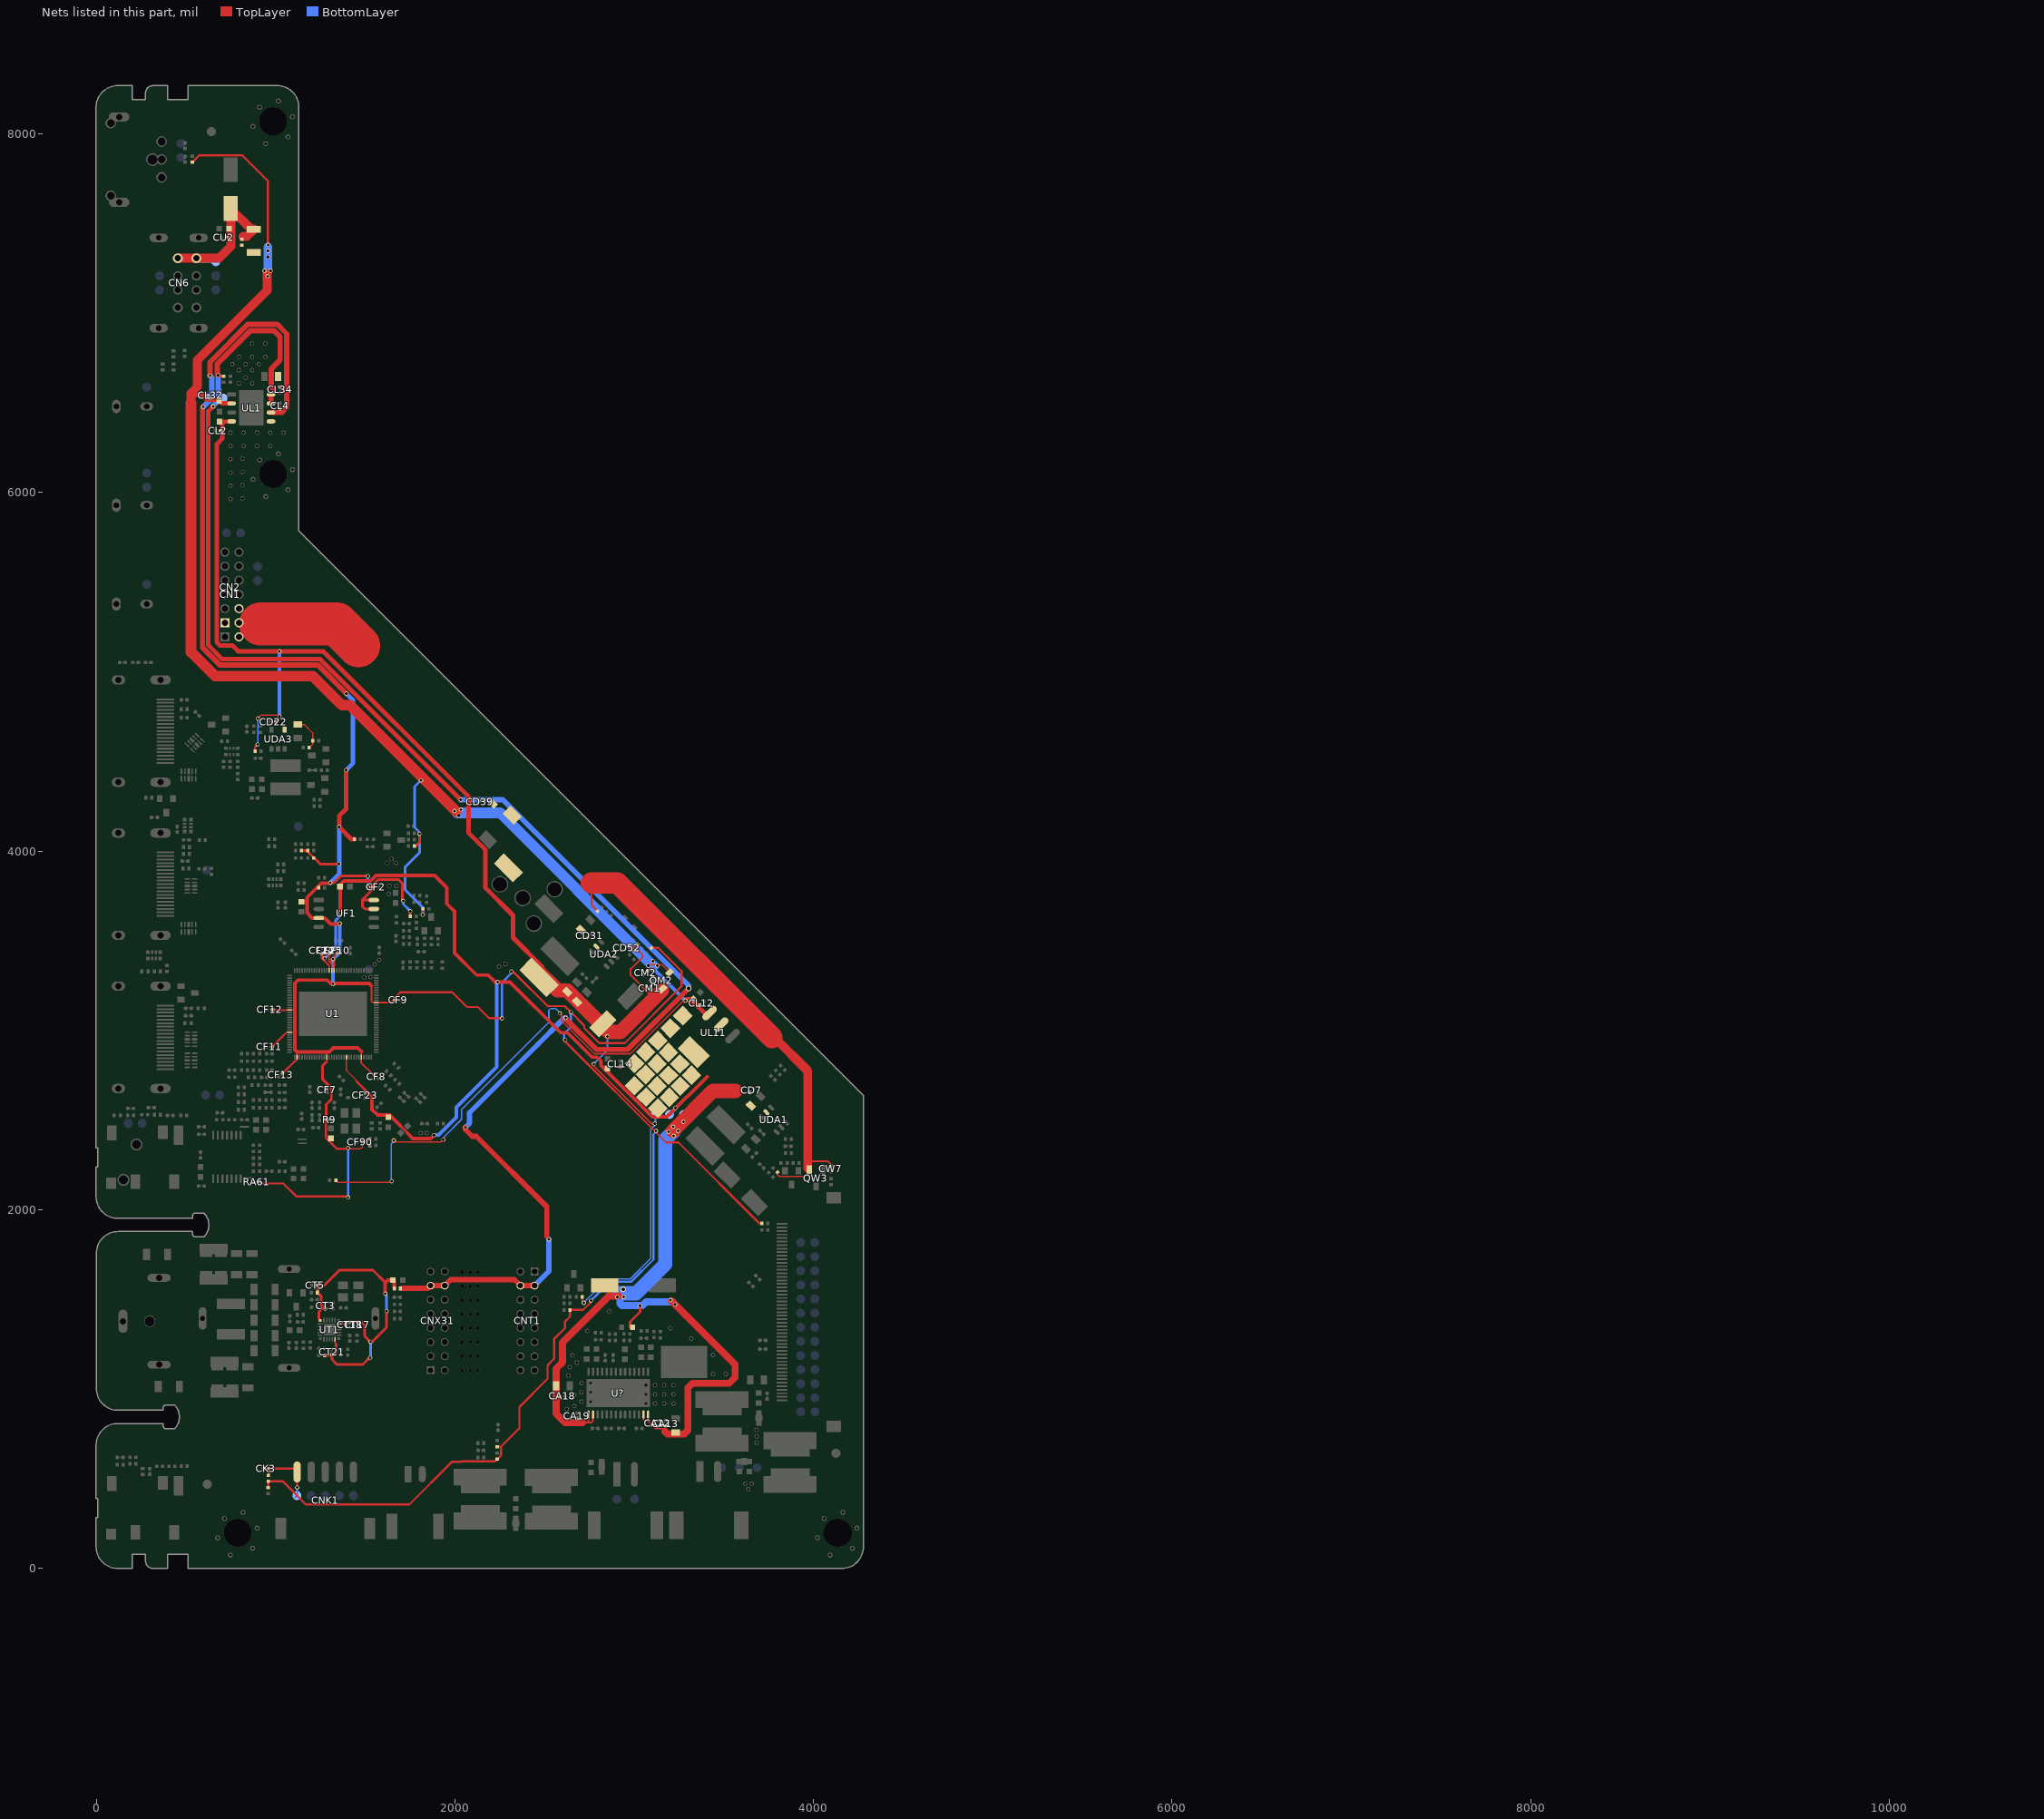
[diagram p0: the nets of this part, all layers, seen from the top]
# Altium PCB MISC105950.PcbDoc (part 5 of 15)
Units mil, origin at the board's own origin, x right, y up, seen from the top; angles counter-clockwise.
Board outline 4280.62 x 8272.76 mil, 2 copper layers (TopLayer, BottomLayer), stack 61.855 mil thick; 541 components, 268 nets, 2324 pads, 1157 vias.

## Part data (continued)
RD43: library part 1K5ohm-0402-±1%-1/16W-D
RD81: library part 10Kohm-0402-±1%-1/16W-D
RD88: library part 12Kohm-0402-±1%-1/16W-D
RF3 RF13 RF29 RF43 RF44 RG3 RG29 RK25 RW13: library part 4K7ohm-0402-±5%-1/16W-D
RF4: library part 100ohm-0402-±5%-1/16W-
RF5: library part 1Kohm-0402-±5%-1/16W-
RF12 RF19 RH101 RH102 RH103 RH104 RH105 RH106: library part 68ohm-0402-±5%-1/16W-D
RFT1: library part XXX.XXX.0005128-D, "RF connector, RF JACK, H, IEC, T14.5, CH6.3, with pipe, 23.8×15.1×11.9mm, SMD, 120-XX1, GD-D"
RG6 RG7 RH72 RH73: library part 33ohm-0402-±5%-1/16W-D
RG8 RG9 RG66 RG67 RH23 RH33 RH70 RK6 RK23: library part 1Kohm-0402-±5%-1/16W-D
RH1 RH74 RH81: library part 22Kohm-0402-±5%-1/16W-D
RH2 RH75 RH82: library part 33Kohm-0402-±5%-1/16W-D
RH24 RH34 RH35 RH71: library part 4*100ohm-0402-±5%-1/16W-D
RH83 RO22 RT1 RT2 RT3 RT4 RT5: library part 004.002.0000568-D, "Thick-film resistor, RES, 1/16W, 100ohm, ±5%, 0402, SMD-D"
RI14 RI16: library part 12Kohm-0402-±5%-1/16W-D
RI21 RI23 RI25 RI36: library part 004.002.0000728-D, "Thick-film resistor, RES, 1/16W, 75ohm, ±5%, 0402, SMD-D"
RI22 RI24 RI26 RI38: library part 004.002.0000658-D, "Thick-film resistor, RES, 1/16W, 33ohm, ±5%, 0402, SMD-D"
RI62 RI63: library part 150ohm-0402-±5%-1/16W-D
RK1: library part 33ohm-0402-±5%-1/16W-
RK2: library part 4K7ohm-0402-±1%-1/16W-D
RK13: library part 004.002.0000663-D, "Thick-film resistor, RES, 1/16W, 33Kohm, ±5%, 0402, SMD-D"
RK14: library part 004.002.0000699-D, "Thick-film resistor, RES, 1/16W, 510ohm, ±1%, 0402, SMD-D"
RL31: library part 004.002.0000584-D, "Thick-film resistor, RES, 1/16W, 120ohm, ±1%, 0402, SMD-D"
RL32: library part 004.002.0000616-D, "Thick-film resistor, RES, 1/16W, 200ohm, ±1%, 0402, SMD-D"
RO21: library part 004.002.0000609-D, "Thick-film resistor, RES, 1/16W, 180ohm, ±5%, 0402, SMD-D"
RO31 RU1: library part 004.002.0000558-D, "Thick-film resistor, RES, 1/16W, 0ohm, ±5%, 0402, SMD-D"
RW12: library part 47Kohm-0402-±5%-1/16W-D
U1: library part 004.016.0001146-D, "TV main IC,IC Main Chip,TSUMV53RWUT-Z1,32bit,Single-Core,QFN128,SMD,Mstar-D"
U?: library part 004.012.0000328-D, "Audio amplifier, IC Audio, Class D, 2x10W@13V@8ohm, HTSSOP-28, SMD, CS3817EO, SEMICO-D"
UA61: library part 004.012.0000155-D, "Audio amplifier, IC Headphone AMP, Class AB, 2×20mW@2.3V@32ohm, TSSOP-14, SMD, AD22653B-QH14NAR, ESMT-D"
UDA1 UDA2: library part 004.010.0001028-D, "DC-DC IC, IC DC-DC, Syn, 2A, 18V, 500kHz, SOT23-6, SMD, SY8120IABC, Silergy-D"
UDA3: library part "DC-DCоƬ,IC DCDC,Syn,1.2A,7.0V,1.5MHz,SOT23-5,SMD,LC2127CB5TR,Leadchip-D"
UF1: library part "SPI FLASH оƬ,IC SPI FLASH,32Mb,SOIC8,SMD,GD25Q32CSIG,GigaDevice-D"
UH1 UH2 UH21 UH22 UH70 UH71: library part ULC0524P-D, "RCLAMP0524J"
UL1: library part 004.010.0000467-D, "LDO IC, IC LDO, 1A, 3.3V+ADJ, 12V, ESOP-8, SMD, LC1118CS8TRAD33, Leadchip-D"
UL11: library part 004.010.0000061-D, "LDO IC, IC LDO, 1A, 1.8V, 12V, SOT-223, SMD, LC1117CLTR18, Leadchip-D"
UT1: library part 004.014.0000255-D, "Silicon tuner IC, IC Si Tuner, QFN-24, SMD, ATBM253, AltoBeam-D"
YF1 YF11: library part 16.000MHz±20PPM-10PF-SMD3225-D
用U1上: library part Φ12mm×12mm-黑色-125度(UL认证)-D

## Free pads (board coordinates)
  round 59.06 on Keep-Out: 0(141.73,8385.83) 0(772.47,8297.25) 0(851.21,8297.25) 0(929.13,8385.83) 0(929.95,8297.25) 0(1155.51,7643.46) 0(1155.51,7879.68) 0(1155.51,7564.72) 0(1155.51,7800.94) 0(1155.51,7722.2) 0(1728.21,5224.54) 0(1783.88,5168.86) 0(1839.56,5113.18) 0(1895.24,5057.5) 0(1950.92,5001.83) 0(3509.72,3443.06) 0(3565.39,3387.38) 0(3621.07,3331.71) 0(3676.75,3276.03) 0(3732.43,3220.35) 0(4305.12,722.69) 0(4305.12,565.21) 0(4305.12,643.95) 0(4305.12,801.43) 0(4305.12,880.17) 0(4530.68,147.64) 0(4531.5,59.06) 0(4609.42,147.64) 0(4688.16,147.64) 0(5318.9,59.06)
  round 137.8 on Keep-Out: 0(1495.5,4289) 0(2460.63,767.72) 0(4081,2463.31)
  round 19.68 hole 19.68 unplated: 0(2040.86,1101.41) 0(2040.86,1180.15) 0(2040.86,1258.89) 0(2040.86,1337.63) 0(2040.86,1416.37) 0(2040.86,1495.11) 0(2040.86,1573.85) 0(2040.86,1652.59) 0(2084.17,1101.41) 0(2084.17,1180.15) 0(2084.17,1258.89) 0(2084.17,1337.63) 0(2084.17,1416.37) 0(2084.17,1495.11) 0(2084.17,1573.85) 0(2084.17,1652.59) 0(2127.48,1101.41) 0(2127.48,1180.15) 0(2127.48,1258.89) 0(2127.48,1337.63) 0(2127.48,1416.37) 0(2127.48,1495.11) 0(2127.48,1573.85) 0(2127.48,1652.59)
  rect 78.74x78.74 smd rot 45 mask+0: HS60(3000,2691) HS60(3001,2815) HS60(3063,2753) HS60(3064,2879) HS60(3065,2627) HS60(3127,2689) HS60(3127,2813) HS60(3131,2942) HS60(3131.33,2565.12) HS60(3190.33,2876.24) HS60(3191,2749) HS60(3195,2626) HS60(3201,3011) HS60(3254.36,2812.21) HS60(3256,2688) HS60(3270.39,3081.36) HS60(3319,2750)
  round 23.62 hole 15.75 paste-15.75 mask-15.75: VIA5(594.19,6476.95) VIA5(632.5,6651.5) VIA5(649.63,6480.63) VIA5(677.31,6654) VIA5(747,5964) VIA5(747,6038) VIA5(747,6112) VIA5(747,6186) VIA5(747,6260) VIA5(747,6334) VIA5(757.5,6716) VIA5(793.5,6609) VIA5(793.5,6683) VIA5(793.5,6757) VIA5(813.5,5967) VIA5(813.5,6041) VIA5(813.5,6115) VIA5(813.5,6189) VIA5(821,6260) VIA5(821,6334) VIA5(831.5,6642) VIA5(831.5,6716) VIA5(867.5,6609) VIA5(867.5,6683) VIA5(867.5,6757) VIA5(867.5,6831) VIA5(895,6260) VIA5(895,6334) VIA5(905.5,6716) VIA5(936.6,7237.2) VIA5(941.5,6757) VIA5(941.5,6831) VIA5(953.5,7207.4) VIA5(955.5,7314.1) VIA5(955.7,7348.3) VIA5(955.9,7382.3) VIA5(969,6260) VIA5(969,6334) VIA5(970.5,7237.3) VIA5(1043,6334) VIA5(1494,3295.26) VIA5(1528,3297) VIA5(1551.5,3368.5) VIA5(1576.5,3392.5) VIA5(1621,3933) VIA5(1630.75,3760) VIA5(1634,3806) VIA5(1646,3956) VIA5(1671.5,3933.5) VIA5(1672,3805) VIA5(1807.5,2426.5) VIA5(1842,2426.5) VIA5(1997,4223.5) VIA5(2021,4199) VIA5(2032.5,4231) VIA5(2245.12,3355.62) VIA5(2281.5,3370) VIA5(2616.5,3069.5) VIA5(2622.57,886.29) VIA5(2632.07,1073.5) VIA5(2639.5,1120) VIA5(2654,1186.93) VIA5(2665.57,966.5) VIA5(2665.86,903) VIA5(2679,1145.43) VIA5(2704.98,928.64) VIA5(2704.98,980.07) VIA5(2704.98,1031.51) VIA5(2737.5,1322.93) VIA5(2756.41,928.64) VIA5(2756.41,980.07) VIA5(2756.41,1031.51) VIA5(2860.15,1431.85) VIA5(2904.5,1511.5) VIA5(2940.5,1512) VIA5(3064,917.67) VIA5(3064,969.1) VIA5(3064,1020.53) VIA5(3079,3361) VIA5(3104,3337) VIA5(3104,3385) VIA5(3115.43,917.67) VIA5(3115.43,969.1) VIA5(3115.43,1020.53) VIA5(3128,3361) VIA5(3166.87,917.67) VIA5(3166.87,969.1) VIA5(3166.87,1020.53) VIA5(3190.5,2433) VIA5(3201,1337) VIA5(3202.5,1495) VIA5(3216.5,2461.5) VIA5(3218.3,917.67) VIA5(3218.3,969.1) VIA5(3218.3,1020.53) VIA5(3219.5,2411) VIA5(3227.5,1470.5) VIA5(3244,2438.5) VIA5(3285.51,3165.77) VIA5(3318,1280) VIA5(3439,1188.5) VIA5(3439.21,1082.36) VIA5(3511,1082) VIA5(3618.4,470.2) VIA5(3636.5,439.9) VIA5(3654.5,470.5) VIA5(3681.8,699.2) VIA5(3682,770) VIA5(3682.5,734.3)
  round 92 hole 78.74 unplated: VIA5(2250,3814.5) VIA5(2377,3738) VIA5(2439.5,3595.5) VIA5(2555.5,3786.5)
  round 31.5 hole 19.68 paste-15.75 mask-15.75: VIA5(2938,1554.5) VIA5(3302.75,3233.75)

## Via types
v1: diameter 23.62, hole 15.75, TopLayer to BottomLayer, tented both sides, 1087 vias
v2: diameter 23.62, hole 15.75, TopLayer to BottomLayer, 51 vias
v3: diameter 27.56, hole 19.68, TopLayer to BottomLayer, 15 vias
v4: diameter 31.5, hole 19.68, TopLayer to BottomLayer, tented both sides, 4 vias

## Nets (pads, with @x,y where several pads share a name; then routed paths per layer and width w, separated by ;. In a path a pad name is that pad's centre, name@x,y a point inside that pad or via, vN(x,y) a via of type N, cw(c..) or ccw(c..) an arc to the next point about the centre after c; other vN are vias at no path point)
3V3_IR: 5V_IR.1 CK3.1 CNK1.1 RK1.2 | length 363.6
  TopLayer w12: RK1.2@958,516.73 961.73,520.46 CK3.1@961.73,554.5 1099.41,554.5 CNK1.1@1118.42,535.5 ; CNK1.1@1107.41,546.5 CNK1.1@1118.42,535.5 ; v1(1118.42,448.92) CNK1.1@1118.42,535.5
  BottomLayer w12: 5V_IR.1@1108.02,394.38 5V_IR.1@1117.52,403.88 ; 5V_IR.1@1118.42,404.78 v1(1118.42,448.92)
3V3_STB: 3V3_STB.1 CF2.2@1541.26,3798 CF2.2@1548.15,3798 CF5.2 CF6.2 CF7.2@1285.5,2678 CF7.2@1285.5,2684.89 CF8.2@1549.67,2753.33 CF8.2@1554.54,2748.46 CF9.2@1664.76,3168.5 CF9.2@1671.65,3168.5 CF10.2@1341.5,3427.6 CF10.2@1341.5,3434.49 CF11.1 CF12.2@975.34,3115.5 CF12.2@982.23,3115.5 CF13.2@1033.46,2758.96 CF13.2@1038.33,2763.83 CF90.1 CL4.1 CL10.1 pad.VIA5@594.19,6476.95 pad.VIA5@632.5,6651.5 R9.2 R9.3 RA51.2 RA61.1 RF3.2 RF4.2 RF29.2 RF43.1 RF44.1 RG29.2 RH101.2 RH104.2 RH106.2 RK1.1 RK2.2 RK13.2 RK25.2 RM1.2 U1.15 U1.24 U1.34 U1.46 U1.60 U1.85 U1.112 UF1.3 UF1.7 UF1.8 UL1.5 UL1.6 | length 18795.1
  TopLayer w7: 1103.12,2824.94 1108.07,2824.94 1118.7,2835.56 U1.34@1118.7,2849.72
  TopLayer w8: 1031.45,3112.55 U1.15@1076.34,3112.55 1105.45,3112.55 ; 1046.95,2975.47 1060.01,2988.53 U1.24@1076.34,2988.53 1103.53,2988.53 ; 1105.5,2882.39 1118.7,2869.19 U1.34@1118.7,2849.72 U1.34@1118.25,2849.27 ; 1268.93,2813.7 1284.05,2828.82 U1.46@1284.05,2849.72 ; 1275.79,2872.5 1284.05,2864.24 ; U1.112@1325.39,3334.04 1325.39,3356.78 ; v1@1399.14,2339.5 1474.5,2339.5 1483.5,2348.5 1483.5,2374.77 1502.23,2393.5 RF43.1@1525.5,2393.5 RF44.1@1525.5,2357.5 ; 1476.96,2830 U1.60@1476.96,2849.72 1476.96,2880.54 ; 1534,3162 1542.11,3153.89 U1.85@1560.66,3153.89 ; U1.85@1560.21,3154.33 U1.85@1560.66,3153.89 ; 1581,3153.89 U1.85@1560.66,3153.89
  TopLayer w10: 1325.61,3357 1325.61,3411.71 CF10.2@1341.5,3427.6 ; 1476.74,2830 1476.74,2818.19 1541.6,2753.33 CF8.2@1549.67,2753.33 ; 1581,3153.89 1639.65,3153.89 1655.26,3169.5
  TopLayer w12: RA61.1@911.77,2155 921.42,2145.35 1041.92,2145.35 1113.58,2073.69 1396.81,2073.69 v1(1403,2067.5) ; RA51.2@957.5,449.23 958,449.73 RK1.1@958,483.27 1039.23,483.27 1055,467.5 ; CF11.1@980,2908.52 1046.95,2975.47 ; CF12.2@982.23,3115.5 985.9,3111.83 1053.83,3111.83 ; CF13.2@1040.43,2762.24 1103.12,2824.94 ; 1049.23,473.27 1055,467.5 ; R9.2@1279.84,2500.5 1279.84,2398.4 1338.74,2339.5 1399.14,2339.5 v1(1402.95,2343.31) ; 1534,3162 1534,3246.88 ; 1655.26,3169.5 1655.26,3170.29 ; CF9.2@1664.76,3168.5 1664.76,3182.5 1694.57,3212.31 1983.89,3212.31 2066.52,3129.68 2127.14,3129.68 2189.12,3067.7 v1@2262,3067.7 ; 2218.73,594.5 2037.24,594.5 2034.46,591.71 1981.88,591.71 1745.04,354.88 1167.62,354.88 1055,467.5 ; 2222.73,594.5 RK25.2@2235.5,607.27 2236.29,607.27 2256.34,627.32 2256.34,642.5 ; RK2.2@2235.5,677.27 2256.03,677.27 2358.5,779.74 2358.5,898.19 2515.86,1055.55 2515.86,1130.85 2551.86,1166.85 2551.86,1277.17 2614,1339.31 2614,1375.3 2640.73,1402.03 RK13.2@2640.73,1440 2714.69,1440 v1@2758.02,1483.33 ; 2256.34,656.43 2256.34,642.5 ; 2256.34,676.95 2256.34,642.5 ; v1@2323.47,3327.12 2516.59,3134 ; 2515.5,3137 2517.5,3135 2612.5,3135 v1(2646.5,3101) 2720.89,3026.61 2720.89,3012.11 2804.11,2928.89 2946.97,2928.89 3263,3244.91 3263,3330.41 3133.74,3459.67 RM1.2@3095.33,3459.67 ; v1@2609.59,2942.27 3177.36,2374.5 3245.4,2374.5 3697.63,1922.27 RF4.2@3708.24,1922.27
  TopLayer w15: RH101.2@1143.16,4002 RH106.2@1177.2,4002 1177.2,3998.13 1247.33,3928 v1(1352,3928) ; 1261.54,2779.35 1261.54,2764.5 ; R9.2@1281.34,2502.43 1281.34,2585.96 1309.81,2614.43 1309.81,2677.44 1261.54,2725.71 1261.54,2764.5 ; 1282.33,2823.56 1261.54,2802.77 1261.54,2764.5 ; CF7.2@1285.5,2684.89 CF7.2@1288.41,2684.89 ; v1(1304,3823) 1324.5,3823 1361.5,3860 v1(1513.5,3860) ; 1487.5,3726.5 UF1.8@1546.59,3726.5 ; v1(1513.5,3798) CF2.2@1540.76,3798 ; 1532,3798 CF2.2@1540.76,3798 ; UF1.7@1540.76,3682.32 UF1.7@1546.59,3676.5 1497.5,3676.5 1484,3690 1484,3730 1541.26,3787.26 CF2.2@1541.26,3798 ; CF2.2@1540.76,3800.5 CF2.2@1540.76,3798 ; v1@1707,3726 1707,3818.52 1684.52,3841 1570.5,3841 1541.26,3811.76 CF2.2@1541.26,3798 ; RF29.2@1749.77,3636.5 1749.77,3664.27 v1(1750,3664.5) ; CF2.2@1540.76,3798 CF2.2@1541.26,3798
  TopLayer w20: CF5.2@1142.5,3717.31 1171.66,3717.31 ; UF1.3@1219.22,3626.5 UF1.3@1239.5,3626.5 ; v1@1300,3821 1254.04,3821 1173.97,3740.93 1173.97,3655.03 1202.5,3626.5 UF1.3@1239.5,3626.5 ; v1@1355.57,3593.81 1306.11,3593.81 1273.42,3626.5 UF1.3@1239.5,3626.5 ; 1476.96,2880.54 1456.5,2901 1320.81,2901 1298.31,2878.5 1118,2878.5 1105.5,2891 1105.5,3261.01 1124.74,3280.26 1285.5,3280.26 1305.5,3260.26 1520.62,3260.26 1531.88,3249
  TopLayer w25: v1(1392.5,4452) 1392.5,4235.48 1353,4195.98 v1(1353,4135) 1422.5,4065.5 RG29.2@1437.77,4065.5
  TopLayer w30: pad.VIA5@591,6476.95 591,5134.54 687.04,5038.5 1233.23,5038.5 v1(1393.28,4878.45) ; pad.VIA5@632.5,6651.5 632.5,6726.51 844.99,6939 1007.5,6939 1060.85,6885.65 1060.85,6569 ; UL1.6@973.05,6447 1032.6,6447 1060.85,6475.25 1060.85,6569 ; 1060.85,6522.82 1060.85,6569
  BottomLayer w12: v1(1402.95,2343.31) v1(1403,2067.5) v1(1403,2067.5) ; v1(2262,3066.5) 2262,3267 v1@2314.76,3319.76 ; v1@2608.5,2949.5 2608.5,2981.5 2646.5,3019.5 v1(2646.5,3101) ; v1@2613.08,2947 v1(2613.7,2946.37) ; v1(2758.02,1491.55) 2864.47,1598 2983.71,1598 3107,1721.29 3107,2419.5 v1@3121.22,2433.72
  BottomLayer w15: v1(1513.5,3798) v1(1513.5,3860) ; v1(1710.5,3722.5) 1710.5,3704 v1(1750,3664.5) v1@1745.4,3664.5
  BottomLayer w20: v1@1318.8,3258.7 v1(1318.8,3397.46) 1355.57,3434.23 v1@1355.57,3593.81
  BottomLayer w25: v1(1304,3823) 1353,3872 v1(1353,4135) ; v1(1392.5,4452) 1431,4490.5 1431,4840.73 v1(1393.28,4878.45)
  BottomLayer w30: pad.VIA5@594.19,6476.95 642.31,6525.08 642.31,6641.69 pad.VIA5@632.5,6651.5
  other v1: 3121.22,2438.86 1319.5,3258 2314.76,3327.12 1357.38,3595.62
3V3_TUN: CT3.2@1276,1446.26 CT3.2@1276,1453.15 CT5.1 CT17.1 CT18.2@1412.5,1367.35 CT18.2@1412.5,1374.24 CT21.2@1313,1188.76 CT21.2@1313,1195.65 CT80.2 FT2.2 LT1.2 RT1.1 UT1.6 UT1.12 UT1.19 | length 1900.3
  TopLayer w7: UT1.6@1331,1268.18 UT1.6@1331,1276.85 ; UT1.6@1331,1277.85 UT1.6@1331,1276.85 ; 1337,1248.67 1337,1249.5 1331,1255.5 UT1.6@1331,1276.85
  TopLayer w7.8: UT1.12@1352.65,1361.5 1378.5,1361.5
  TopLayer w15: UT1.19@1248.5,1380.98 1241.19,1388.3 1241.19,1429.57 1255.43,1443.81 CT3.2@1268.73,1446.26 ; RT1.1@1272.23,1185.5 1309.74,1185.5 CT21.2@1313,1188.76 ; CT3.2@1276,1453.15 1266.2,1453.15 1253.66,1465.69 1253.66,1514.13 FT2.2@1230.95,1536.84 1234.23,1540.12 CT5.1@1234.23,1577 1271.11,1577 1355.61,1661.5 1541,1661.5 1610.5,1592 ; 1337,1248.67 1337,1196.5 1329.26,1188.76 CT21.2@1313,1188.76 ; 1380,1363 1382,1363 1393.23,1374.23 CT17.1@1455,1374.23 1471.77,1374.23 ; 1474.77,1374.23 1495.5,1353.5 1495.5,1293.5 v1(1528,1261) ; v1@1521.5,1172 1485.19,1135.69 1340.31,1135.69 1313,1163 CT21.2@1313,1188.76 ; v1@1536.14,1261 1618,1342.86 v1(1618,1432.5) v1@1618,1432.87
  TopLayer w20: v1(1610.5,1530) 1610.5,1592 1624,1605.5 CT80.2@1653.19,1605.5 1659.5,1605.5 1659.5,1561.26 LT1.2@1660.76,1560
  BottomLayer w15: v1@1528,1174 v1(1528,1261) ; v1(1618,1432.5) v1@1618,1522.5
  other v1: 1526,1172
3V3_TUN_OUT: 3V3_Tun.1 CL34.2@1023.5,6584.34 CL34.2@1023.5,6591.23 CNT1.3 CNT1.4 CNX31.13 CNX31.14 LT1.1 pad.VIA5@649.63,6480.63 pad.VIA5@677.31,6654 pad.VIA5@2616.5,3069.5 pad.VIA5@3302.75,3233.75 RL31.2 UL1.7 UL1.8 | length 9535.3
  TopLayer w15: pad.VIA5@677.27,6653.73 pad.VIA5@677.16,6653.84 ; pad.VIA5@677.31,6654 677,6654 pad.VIA5@677.16,6653.84 ; RL31.2@709.5,6648.73 682.27,6648.73 pad.VIA5@677.16,6653.84
  TopLayer w25: pad.VIA5@649.63,6480.63 623.5,6454.5 623.5,5148 700.5,5071 1246.69,5071 v1(2031.19,4286.5)
  TopLayer w30: pad.VIA5@677,6654 672.5,6658.5 672.5,6717.01 859.49,6904 988.5,6904 1024,6868.5 1024,6740 975.32,6691.31 975.32,6593 ; UL1.7@973.05,6504 UL1.8@973.05,6547 ; 975.32,6589.11 987.03,6577.39 ; LT1.1@1703,1560 1847.78,1560 CNX31.13@1863.21,1575.43 CNX31.14@1941.95,1575.43 1975.52,1609 2330.84,1609 CNT1.4@2364.47,1575.37 CNT1.3@2443.21,1575.37 CNT1.3@2443.21,1582.52 ; v1(2057.95,2457.99) 2057.95,2446.54 2095.99,2408.5 2117.99,2408.5 2511.81,2014.67 2511.81,1850.5 ; pad.VIA5@2616.5,3065.5 2789.11,2892.89 2961.89,2892.89 pad.VIA5@3302.75,3233.75
  BottomLayer w30: pad.VIA5@649.63,6480.63 649.63,6482.9 677.31,6510.58 pad.VIA5@677.31,6654 ; v1(2031.19,4286.5) 2266.22,4286.5 3302.75,3249.97 pad.VIA5@3302.75,3233.75 ; v1(2057.95,2457.99) 2080.67,2480.71 2080.67,2540.03 2462.82,2922.19 2590.57,3049.93 2610.13,3069.5 pad.VIA5@2616.5,3069.5 ; CNT1.3@2443.21,1575.37 2523.15,1655.31 v1(2523.15,1833.15)
5V_M: CL11.2 CL12.2@3364.17,3138.67 CL12.2@3369.04,3143.54 CL31.1 CL32.1 CM2.2@3068.46,3326.96 CM2.2@3073.33,3331.83 FU1.2 pad.VIA5@936.6,7237.2 pad.VIA5@953.5,7207.4 pad.VIA5@955.5,7314.1 pad.VIA5@955.7,7348.3 pad.VIA5@955.9,7382.3 pad.VIA5@970.5,7237.3 pad.VIA5@1997,4223.5 pad.VIA5@2021,4199 pad.VIA5@2032.5,4231 pad.VIA5@3079,3361 pad.VIA5@3104,3337 pad.VIA5@3104,3385 pad.VIA5@3128,3361 pad.VIA5@3285.51,3165.77 QM2.D RA70.2 RG66.2 RG67.2 RO31.2 RU1.2 UL1.2 UL11.3 | length 11181.6
  TopLayer w8: RA70.2@1334.23,2162.5 1345.04,2151.69 v1@1640.69,2151.69 ; v1@1660.5,2377.5 1922.5,2377.5 v1(1934.5,2389.5) ; v1@2592.5,3087.5 2592.5,3053.5 2777.11,2868.89 2976.89,2868.89 2978.5,2870.5 ; 2979,2870.5 2978.5,2870.5 ; CM2.2@3075.33,3333.83 3086.29,3344.79 pad.VIA5@3106.21,3344.79 ; pad.VIA5@3085,3366 3154.03,3366 QM2.D@3190.01,3330.02 ; pad.VIA5@3280.9,3172.9 2978.5,2870.5 ; CL11.2@3311.77,3172.9 CL11.2@3320.33,3164.33 ; CL11.2@3323.83,3166.83 3328.33,3166.83 CL11.2@3336,3166.83 ; UL11.3@3401.24,3095.59 UL11.3@3420.03,3095.59
  TopLayer w12: RO31.2@534,7842.65 534.79,7842.65 554.84,7862.7 554.84,7863.49 572.52,7881.17 813.05,7881.17 955.9,7738.31 pad.VIA5@955.9,7382.3
  TopLayer w15: RG66.2@1777.73,4025.5 1801.5,4049.27 v1@1801.5,4101 ; v1@1821.27,3645.77 RG67.2@1821.27,3677.5
  TopLayer w25: 527,6554 537.46,6543.54 587.46,6543.54 613.5,6517.5 635.43,6517.5 677.88,6517.5 CL31.1@683.93,6511.45 698.38,6497 UL1.2@753.95,6497 ; pad.VIA5@3285.51,3165.77 3293.08,3173.33 CL11.2@3328.33,3173.33 3328.33,3166.83 3328.33,3159.77 3392.51,3095.59 UL11.3@3420.03,3095.59
  TopLayer w50: 527,6501.5 527,6554 562.5,6589.5 562.5,6738.53 951.5,7127.53 pad.VIA5@951.5,7218.5
  TopLayer w60: 527,6501.5 527,5109.44 660.94,4975.5 1207.13,4975.5 1307.57,4875.07 ; 1307.57,4874.59 1368.28,4813.87 1413.97,4813.87 2003.28,4224.56 2008.35,4219.5
  BottomLayer w8: v1@1643.5,2165.5 1643.5,2367 v1@1657.5,2381 ; v1@1934.5,2400.56 2036.67,2502.73 2036.67,2558.26 2523.41,3045 2523.41,3111.41 2533.5,3121.5 2560.43,3121.5 2585,3096.93 v1(2585,3095)
  BottomLayer w15: v1(1809.5,4394.5) 1774,4359 1774,4131.53 1801.5,4104.03 1801.5,3991 1721.5,3911 1721.5,3784 1820,3685.5 v1(1820,3644.5)
  BottomLayer w20: pad.VIA5@3106.21,3344.79 pad.VIA5@3285.37,3165.63
  BottomLayer w50: 955.46,7239.36 955.46,7369.4
  BottomLayer w60: 2011.5,4213.5 2250.12,4213.5 3104.56,3359.06
  other v1: 1646.5,2157.5 1657.5,2385.5 1801.5,4095.5
5V_STB: 5V_STB.1 CD22.2@994.5,4721.5 CD22.2@1001.39,4721.5 CD52.2@2963.68,3467.07 CD52.2@2968.55,3471.94 CD53.1 CD54.1 CD57.1 CL1.2 CL2.2@687.85,6345 CL2.2@694.74,6345 CM1.2@3089.66,3227.13 CM1.2@3094.53,3222.26 EA1.1 LD11.2 QM2.S RD2.1 RD42.2 RD43.2 RD91.2 RK10.2 RM3.2 UDA3.4 UL1.4 | length 8410
  TopLayer w8: v1(899.5,4739.5) 917.34,4757.34 1014.16,4757.34 v1(1021,4750.5) ; CD54.1@1123,4706 1157.5,4706 1205.27,4658.23 RD42.2@1205.27,4615 1205.27,4594.77 RD43.2@1187,4576.5 ; 2709.23,1488.77 RK10.2@2709.23,1512.5
  TopLayer w10: RD2.1@883.54,4556.5 883.54,4581.04 v1@897.25,4594.75 ; v1@2773,2801.49 3095.49,2479 v1(3114.5,2479) ; EA1.1@2825.69,2997.69 EA1.1@2827.5,2997.69 ; CD52.2@2968.55,3471.94 2996.05,3444.43 RD91.2@2996.55,3444.43 ; RM3.2@3017.33,3477.17 2996.55,3456.39 RD91.2@2996.55,3444.43 ; 3082.25,3204.75 2979,3308 2979,3341.44 3045.06,3407.49 3045.06,3421.28 3022.07,3444.27 3022.07,3444.43 RD91.2@2996.55,3444.43 ; CM1.2@3088.83,3221.67 CM1.2@3088.83,3224.17
  TopLayer w25: UL1.4@753.95,6397 752.64,6395.69 CL1.2@685.5,6395.69 700.5,6380.69 700.5,6299.5 670.5,6269.5 670.5,5164.28 687.28,5147.5 757.09,5147.5 790.59,5114 1264.5,5114 2076,4302.5 2076,4100.3 2169.5,4006.8 2169.5,3794.8 2323.5,3640.8 2323.5,3516.91 2486.4,3354.01
  TopLayer w80: LD11.2@2452,3342.5 2572,3222.5 2626.39,3222.5 2859,2989.89 2921.71,2989.89 QM2.S@3153.41,3221.59
  BottomLayer w8: v1@899.5,4595.5 v1(899.5,4739.5) ; v1(2718,1480) 2718,1480.96 2850.04,1613 2977.5,1613 3092,1727.5 3092,2447.5 v1@3114.5,2470
  BottomLayer w10: v1(2773,2811.5) 2849,2887.5 v1(2849,2966) ; v1@3117,2481.5 5V_STB.1@3117,2530.5
  BottomLayer w20: v1(1021,4750.5) v1(1021,5113.5)
  other v1: 898,4594
5V_USB2.0: 5V.1 CN6.1 CN6.5 CU1.2 CU2.1 EU1.1 FU1.1 RU1.1 | length 1003.3
  TopLayer w50: CN6.5@453.15,7307.09 612,7307.09 ; 669.71,7307.09 612,7307.09 ; EU1.1@747,7584.73 EU1.1@750,7581.73 ; EU1.1@750,7624.61 EU1.1@750,7581.73 ; 818,7429 837.42,7429 FU1.1@877.38,7468.96 862.77,7468.96 EU1.1@750,7581.73 ; 612,7307.09 682.59,7307.09 750,7374.5 750,7533.5 EU1.1@750,7581.73
  BottomLayer w12: CN6.1@556.3,7307.09 575.27,7288.12 5V.1@664.87,7288.12
12V/15V: 12V/15V.1 CA1.2 CA2.2 CA12.2@3130.5,789.76 CA12.2@3130.5,796.65 CA13.2@3173,789.43 CA13.2@3173,796.31 CA18.2@2581.76,958.5 CA18.2@2588.65,958.5 CA19.2@2680,831.76 CA19.2@2680,838.65 CD7.1 CD30.2 CD31.1 CD39.1 CD77.2 CD96.2 CN1.2 CN1.3 CN1.4 CN1.6 CN2.1 CN2.2 CN2.4 CW7.2@4095.5,2236.85 CW7.2@4095.5,2243.74 DM4.K EA33.1 EA34.1 pad.VIA5@2904.5,1511.5 pad.VIA5@2938,1554.5 pad.VIA5@2940.5,1512 pad.VIA5@3190.5,2433 pad.VIA5@3202.5,1495 pad.VIA5@3216.5,2461.5 pad.VIA5@3219.5,2411 pad.VIA5@3227.5,1470.5 pad.VIA5@3244,2438.5 QW3.S RA7.1 RD52.1 RW10.2 U?.15 U?.16 U?.27 U?.28 UDA1.5 UDA2.5 | length 8108.2
  TopLayer w7: U?.27@3050.95,854.34 3050.95,830.05 3061,820 3076.53,820 3119.76,776.76 3128,776.76 3171.5,776.76 3172,776.26 ; 3076.54,822.04 U?.28@3076.54,854.34
  TopLayer w8: RW10.2@3798.33,2207.67 3798.33,2194.67 3808.69,2184.31 3948.32,2184.31
  TopLayer w10: 2710.75,811.75 2743,811.75 ; U?.15@2743.87,854.34 2743.87,812.62 2743,811.75 ; 2761.3,3799.5 2761.3,3698.54 RD52.1@2795.92,3663.92 ; 2761.3,3822 2761.3,3845.8 ; U?.16@2769.46,854.34 2769.46,819.96 2761.25,811.75 2743,811.75 ; 3967.1,2270 4078.5,2270 4095.5,2253 CW7.2@4095.5,2236.85
  TopLayer w15: RA7.1@2976.95,1343.22 2976.23,1342.5 2976.23,1372.81 3032.31,1428.88 v1(3032.31,1463)
  TopLayer w40: 2710.75,811.75 2613.75,811.75 2562.86,862.64 2562.86,1111.38 2598.86,1147.38 2598.86,1257.7 2858.16,1517 pad.VIA5@2913,1517 ; 3172,760 3185.03,746.97 3276.97,746.97 3298.86,768.86 3298.86,907 ; pad.VIA5@3207.58,1489.58 3288.58,1408.58 ; 3245.66,1451.5 3288.58,1408.58 ; 3298.86,830.86 3298.86,907 ; 3298.86,853.86 3298.86,907 ; 3288.58,1408.58 3562,1135.16 3562,1063.29 3529,1030.29 3324.05,1030.29 3298.86,1005.1 3298.86,907
  TopLayer w50: 3767.82,2960.13 3781.32,2960.13 3967.1,2774.34 3967.1,2270 QW3.S@3967.1,2231.08
  TopLayer w80: 3216.49,2439.5 3438.99,2662 3565,2662
  TopLayer w120: 2761.3,3822 2905.95,3822 3767.82,2960.13
  TopLayer w240: 915.5,5267.5 1340.41,5267.5 1462.47,5145.44 1462.47,5144.62
  BottomLayer w10: v1(3274.48,2489.02) 12V/15V.1@3274.48,2530.5
  BottomLayer w40: 2921,1533 2921,1475 2931,1465 3045.5,1465 3065.5,1485 3215,1485
  BottomLayer w80: 2921,1533 3010.64,1533 3172,1694.36 3172,2389.5 3216,2433.5
+1.8V_DDR: 1V8_DDR.1 CF3.2 CF23.2@1497,2647.34 CF23.2@1497,2654.23 CF24.2@1257,3427.6 CF24.2@1257,3434.49 CF25.1 CF58.2 CL13.2 CL14.2@2921.5,2796.26 CL14.2@2921.5,2803.15 pad.HS60 U1.54 U1.113 U1.114 UL11.2 UL11.4 | length 5434.7
  TopLayer w8: 1291.6,3369.1 1297.83,3362.88 U1.114@1297.83,3334.04 ; U1.113@1311.61,3334.04 1311.61,3371.5 ; U1.54@1394.29,2849.72 1394.29,2774.78 1449.72,2719.34 1449.72,2714.39
  TopLayer w12: CF24.2@1257,3427.6 CF25.1@1299.5,3427.61 ; v1@1261.76,3396.82 1289.48,3369.1 ; CF25.1@1301.25,3425.86 CF25.1@1299.5,3427.61 ; 1309.61,3374.39 1303.5,3380.5 1295.99,3388.01 1295.99,3424.1 CF25.1@1299.5,3427.61
  TopLayer w14: 1692.29,2468.29 1699.31,2461.27 ; 1701.15,2461.27 1734.19,2428.23
  TopLayer w15: CF24.2@1257,3427.6 1257,3403.71 1259.78,3400.93 v1@1265.87,3400.93 ; 1449.72,2714.39 1534.81,2629.31
  TopLayer w20: CF3.2@1358.19,3802 1358.19,3654.24 1359,3655.05 v1(1359,3655.5) ; CF3.2@1359,3812 1379.75,3832.75 1528.75,3832.75 1559.5,3863.5 1885.25,3863.5 1954,3794.75 1954,3705.53 1995.81,3663.72 1995.81,3431.81 2119.62,3308 2185.25,3308 2224.75,3268.5 v1(2236.5,3268.5) 2306.38,3268.5 2588.19,2986.69 2626.31,2986.69 2763.11,2849.89 2792.36,2849.89 2815,2827.25 2815,2802.69 3100.69,2517 3182.27,2517 3406.27,2741 ; 1537.31,2623.28 1537.31,2558.78 1569.5,2526.59 1592.68,2526.59 CF58.2@1633.99,2526.59 ; CF58.2@1636.89,2523.7 1692.29,2468.29 ; 1733.27,2427.31 1764.08,2396.5 1864,2396.5 v1(1882,2414.5)
  BottomLayer w15: v1(1272.37,3400.93) 1333.07,3461.63 1333.07,3555 1333.07,3611.5 1359.5,3637.93 v1@1359.5,3655
  BottomLayer w20: v1(1359,3655.5) 1359.5,3655 v1@1361.07,3653.43 ; v1@1882,2415 1907.93,2415 2007.67,2514.74 2007.67,2570.27 2232.95,2795.55 v1@2232.95,3264.95 ; 1V8_DDR.1@3195.74,2530.5 3228.5,2563.26 v1(3228.5,2566.5)